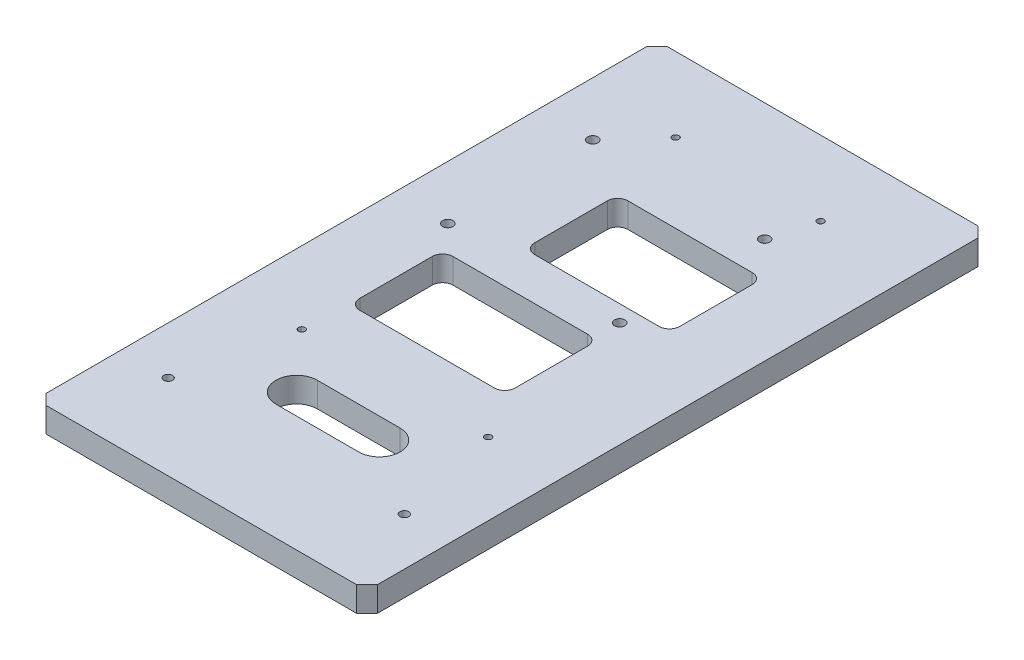
from build123d import *

# Parameters (mm, degrees)
SKETCH_1_W                = 160
SKETCH_1_H                = 300
EXTRUDE_1_DEPTH           = 12
CUT_EXTRUDE_1_DEPTH       = 171.423003142
HOLE_WIZARD_3_D           = 3.2
HOLE_WIZARD_3_CBORE_D     = 6
HOLE_WIZARD_3_CBORE_DEPTH = 7
HOLE_WIZARD_M5_1_D        = 4.2
CHAMFER_1_SIZE            = 5
SKETCH_29_W               = 70
SKETCH_29_H               = 45
SKETCH_29_W_2             = 75
CUT_EXTRUDE_3_DEPTH       = 171.423003142
FILLET_1_R                = 5
HOLE_WIZARD_M6_1_D        = 5


with BuildPart() as part:
    # 草图1 → 凸台-拉伸1 (new body)
    with BuildSketch(Plane(origin=(0, 0, 0), x_dir=(1, 0, 0), z_dir=(0, 1, 0))):
        Rectangle(SKETCH_1_W, SKETCH_1_H)
    extrude(amount=EXTRUDE_1_DEPTH)

    # 草图6 → 切除-拉伸1 (cut, through all)
    with BuildSketch(Plane(origin=(0, 12, 0), x_dir=(1, 0, 0), z_dir=(0, 1, 0))):
        with BuildLine():
            Line((-20, -74), (20, -74))
            ThreePointArc((20, -74), (30, -84), (20, -94))
            Line((20, -94), (-20, -94))
            ThreePointArc((-20, -94), (-30, -84), (-20, -74))
        make_face()
    extrude(amount=-CUT_EXTRUDE_1_DEPTH, mode=Mode.SUBTRACT)

    # Hole Wizard 3 (through all)
    with Locations(Plane(origin=(0, 0, 0), x_dir=(-1, 0, 0), z_dir=(0, -1, 0))):
        with Locations((35, 114), (-35, 114), (45, -56.5), (-45, -56.5)):
            CounterBoreHole(HOLE_WIZARD_3_D / 2, HOLE_WIZARD_3_CBORE_D / 2, HOLE_WIZARD_3_CBORE_DEPTH)

    # M5 螺纹孔1 (through all)
    with Locations(Plane(origin=(0, 12, 0), x_dir=(1, 0, 0), z_dir=(0, 1, 0))):
        with Locations((-57, -109), (57, -109)):
            Hole(HOLE_WIZARD_M5_1_D / 2)

    # 倒角1
    chamfer_1_edges = [part.edges().sort_by_distance(p)[0] for p in [
        (80, 6, 150),
        (-80, 6, 150),
        (-80, 6, -150),
        (80, 6, -150),
    ]]
    chamfer(chamfer_1_edges, length=CHAMFER_1_SIZE)

    # 草图29 → 切除-拉伸3 (cut, through all)
    with BuildSketch(Plane(origin=(0, 12, 0), x_dir=(1, 0, 0), z_dir=(0, 1, 0))):
        with Locations((10, 53.5)):
            Rectangle(SKETCH_29_W, SKETCH_29_H)
        with Locations((-6.5, -12)):
            Rectangle(SKETCH_29_W_2, SKETCH_29_H)
    extrude(amount=-CUT_EXTRUDE_3_DEPTH, mode=Mode.SUBTRACT)

    # 圆角1
    fillet_1_edges = [part.edges().sort_by_distance(p)[0] for p in [
        (31, 6, -10.5),
        (31, 6, 34.5),
        (-44, 6, 34.5),
        (-44, 6, -10.5),
        (45, 6, -76),
        (45, 6, -31),
        (-25, 6, -31),
        (-25, 6, -76),
    ]]
    fillet(fillet_1_edges, radius=FILLET_1_R)

    # M6 螺纹孔1 (through all)
    with Locations(Plane(origin=(0, 12, 0), x_dir=(1, 0, 0), z_dir=(0, 1, 0))):
        with Locations((-54, 93), (29, 93), (-54, 23), (29, 23)):
            Hole(HOLE_WIZARD_M6_1_D / 2)


solid = part.part
